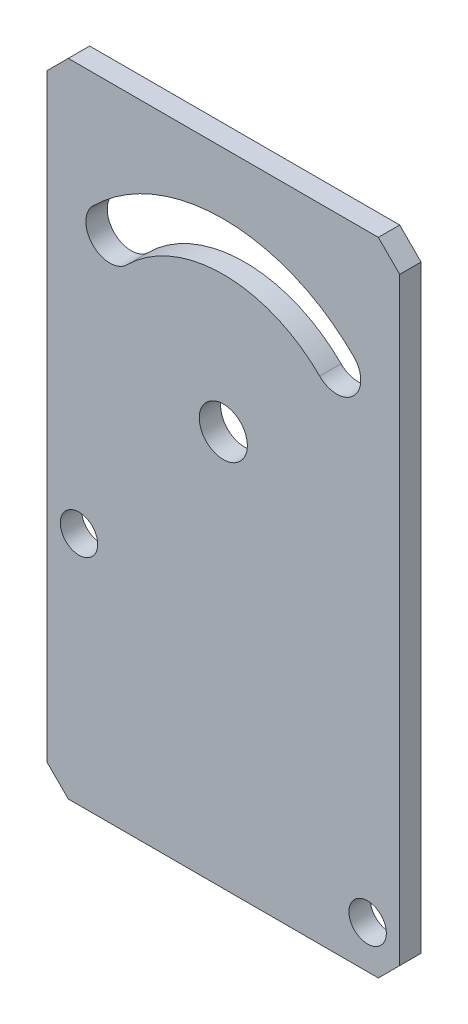
from build123d import *

# Parameters (mm, degrees)
SKETCH1_W           = 33
SKETCH1_H           = 60
SKETCH1_R           = 2.25
SKETCH1_R_2         = 1.75
BOSS_EXTRUDE1_DEPTH = 2
CHAMFER1_SIZE       = 2


with BuildPart() as part:
    # Sketch1 → Boss-Extrude1 (new body)
    with BuildSketch(Plane.XY):
        Rectangle(SKETCH1_W, SKETCH1_H)
        with Locations((0, 7)):
            Circle(SKETCH1_R, mode=Mode.SUBTRACT)
        with Locations((13.5, -26)):
            Circle(SKETCH1_R_2, mode=Mode.SUBTRACT)
        with Locations((-13.5, -8)):
            Circle(SKETCH1_R_2, mode=Mode.SUBTRACT)
        with BuildLine():
            ThreePointArc((9.01561146, 16.01561146), (0, 19.75), (-9.01561146, 16.01561146))
            ThreePointArc((-9.01561146, 16.01561146), (-12.197591975, 16.01561146), (-12.197591975, 19.197591975))
            ThreePointArc((-12.197591975, 19.197591975), (0, 24.25), (12.197591975, 19.197591975))
            ThreePointArc((12.197591975, 19.197591975), (12.197591975, 16.01561146), (9.01561146, 16.01561146))
        make_face(mode=Mode.SUBTRACT)
    extrude(amount=BOSS_EXTRUDE1_DEPTH)

    # Chamfer1
    chamfer1_edges = [part.edges().sort_by_distance(p)[0] for p in [
        (16.5, -30, 1),
        (-16.5, -30, 1),
        (-16.5, 30, 1),
        (16.5, 30, 1),
    ]]
    chamfer(chamfer1_edges, length=CHAMFER1_SIZE)


solid = part.part
